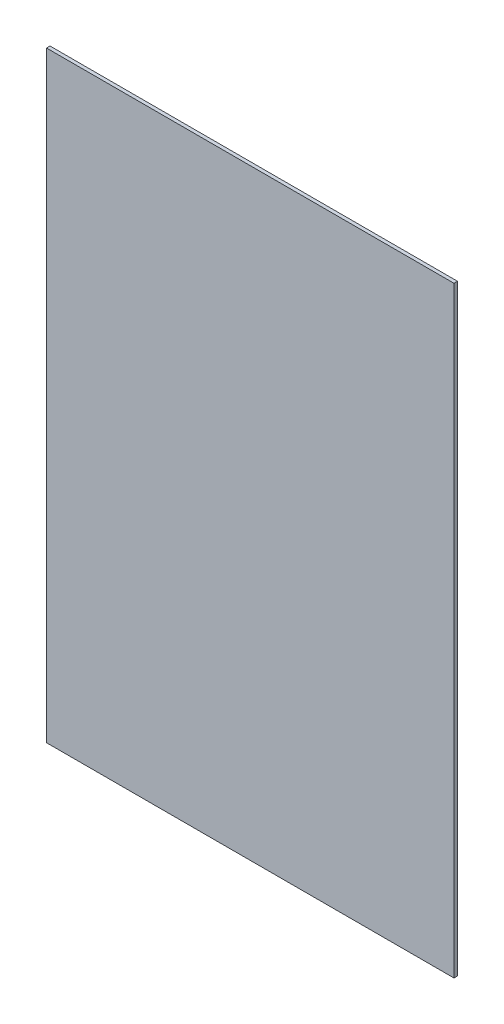
SolidWorks part; units mm, degrees
material "PMMA(有机玻璃)"
ref_plane "前视" through (0, 0, 0) normal (0, 0, 1) x (1, 0, 0)
ref_plane "上视" through (0, 0, 0) normal (0, 1, 0) x (1, 0, 0)
ref_plane "右视" through (0, 0, 0) normal (1, 0, 0) x (0, 0, -1)
sketch "草图1" plane through (0, 0, 0) normal (0, 0, 1) x (1, 0, 0)
  line L1 (-290.5, 429) -> (290.5, 429)
  line L2 (-290.5, 429) -> (-290.5, -429)
  line L3 (-290.5, -429) -> (290.5, -429)
  line L4 (290.5, 429) -> (290.5, -429)
  line L5 (-290.5, 429) -> (290.5, -429) construction
  line L6 (-290.5, -429) -> (290.5, 429) construction
  point P0 (0, 0)
  dimension "D1" = 858
  dimension "D2" = 581
extrude "凸台-拉伸1" add sketch "草图1" along normal blind 5
